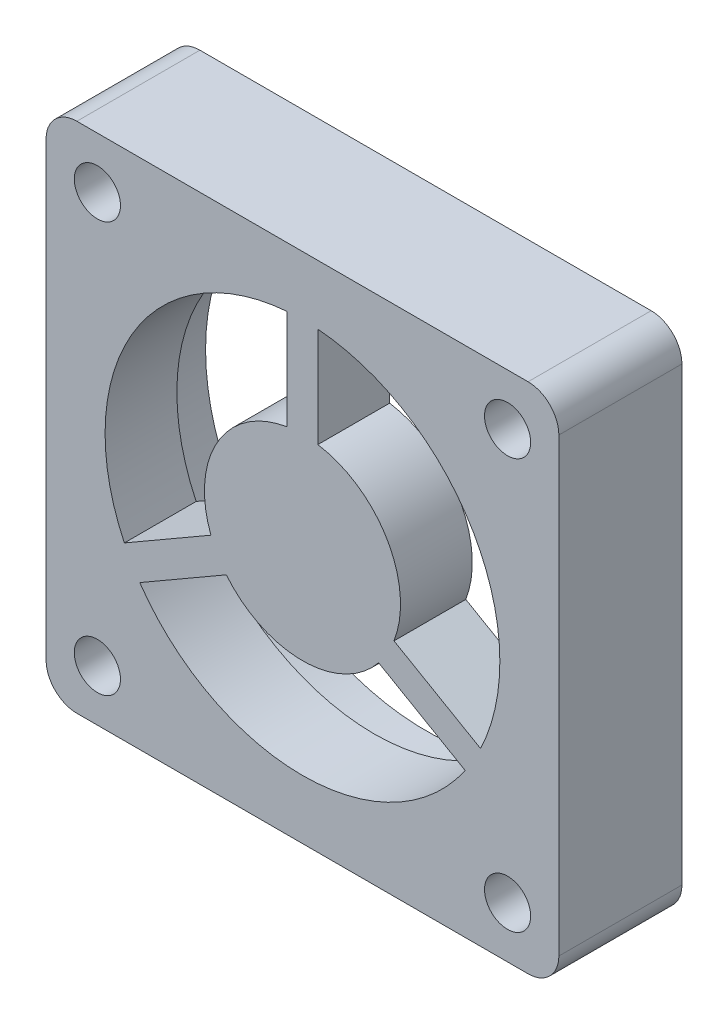
SolidWorks part; units mm, degrees
ref_plane "Front Plane" through (0, 0, 0) normal (0, 0, 1) x (1, 0, 0)
ref_plane "Top Plane" through (0, 0, 0) normal (0, 1, 0) x (1, 0, 0)
ref_plane "Right Plane" through (0, 0, 0) normal (1, 0, 0) x (0, 0, -1)
other "Configuration Table"
sketch "Sketch1" plane through (0, 0, 0) normal (0, 0, 1) x (1, 0, 0)
  line L1 (-22, 25) -> (22, 25)
  line L2 (-25, 22) -> (-25, -22)
  line L3 (-22, -25) -> (22, -25)
  line L4 (25, 22) -> (25, -22)
  line L5 (-25, 25) -> (25, -25) construction
  line L6 (-25, -25) -> (25, 25) construction
  line L7 (-20, -20) -> (20, -20) construction
  line L8 (-20, -20) -> (-20, 20) construction
  line L9 (-20, 20) -> (20, 20) construction
  line L10 (20, -20) -> (20, 20) construction
  line L11 (-20, -20) -> (20, 20) construction
  line L12 (-20, 20) -> (20, -20) construction
  circle A0 centre (-20, 20) radius 2.25
  circle A1 centre (20, 20) radius 2.25
  circle A2 centre (20, -20) radius 2.25
  circle A3 centre (-20, -20) radius 2.25
  arc A4 (22, -25) -> (25, -22) centre (22, -22) ccw
  arc A5 (-25, -22) -> (-22, -25) centre (-22, -22) ccw
  arc A6 (-22, 25) -> (-25, 22) centre (-22, 22) ccw
  arc A7 (22, 25) -> (25, 22) centre (22, 22) cw
  point P0 (0, 0)
  point P6 (0, 0)
  dimension "D5" = 4.5
  dimension "D6" = 3
  dimension "D1" = 50
  dimension "D2" = 50
  dimension "D3" = 40
  dimension "D4" = 40
extrude "Boss-Extrude1" add sketch "Sketch1" along normal blind 12
sketch "Sketch2" plane through (0, 0, 12) normal (0, 0, 1) x (1, 0, 0)
  line L0 (-1.5, 19.1888) -> (-1.5, 9.4407)
  line L1 (1.5, 19.1888) -> (1.5, 9.4407)
  line L2 (17.368, -8.2954) -> (8.9259, -3.4213)
  line L3 (15.868, -10.8934) -> (7.4259, -6.0194)
  line L4 (-15.868, -10.8934) -> (-7.4259, -6.0194)
  line L5 (-17.368, -8.2954) -> (-8.9259, -3.4213)
  arc A0 (-1.5, 19.1888) -> (-17.368, -8.2954) centre (0, 0) ccw
  arc A1 (-1.5, 9.4407) -> (-8.9259, -3.4213) centre (0, 0) ccw
  arc A2 (-15.868, -10.8934) -> (15.868, -10.8934) centre (0, 0) ccw
  arc A3 (-7.4259, -6.0194) -> (7.4259, -6.0194) centre (0, 0) ccw
  arc A4 (8.9259, -3.4213) -> (1.5, 9.4407) centre (0, 0) ccw
  arc A5 (17.368, -8.2954) -> (1.5, 19.1888) centre (0, 0) ccw
  point P16 (0, 0)
  dimension "D1" = 3
  dimension "D2" = 1.5
  dimension "D3" = 3
extrude "Cut-Extrude1" cut sketch "Sketch2" against normal blind 12
sketch "Sketch3" plane through (0, 0, 0) normal (0, 0, -1) x (-1, 0, 0)
  circle A0 centre (0, 0) radius 21.4496
extrude "Cut-Extrude2" cut sketch "Sketch3" against normal blind 5
